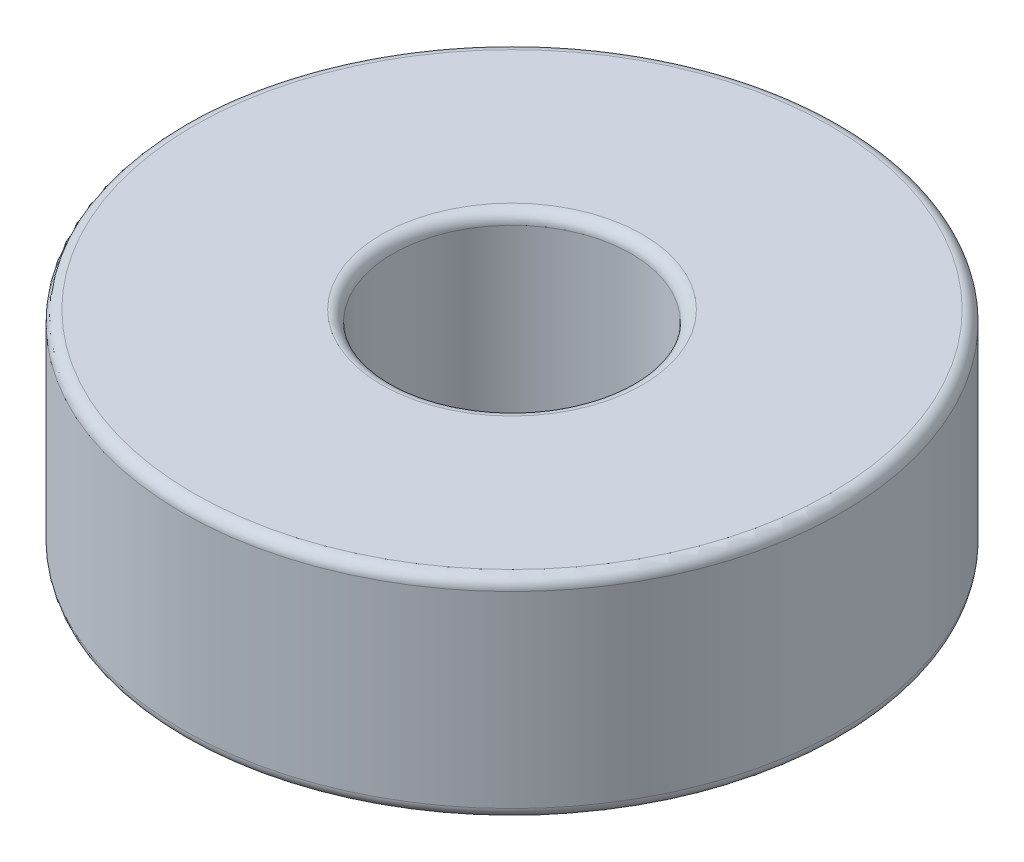
from build123d import *

# Parameters (mm, degrees)
SKETCH_1_R      = 23.5
SKETCH_1_R_2    = 8.5
EXTRUDE_1_DEPTH = 15
FILLET_1_R      = 0.8


with BuildPart() as part:
    # 草图1 → 拉伸1 (new body)
    with BuildSketch(Plane(origin=(0, 0, 0), x_dir=(1, 0, 0), z_dir=(0, 1, 0))):
        with Locations(Location((0, 0, 0), (0, 0, 270))):
            Circle(SKETCH_1_R)
        with Locations(Location((0, 0, 0), (0, 0, 270))):
            Circle(SKETCH_1_R_2, mode=Mode.SUBTRACT)
    extrude(amount=EXTRUDE_1_DEPTH)

    # 圆角1
    fillet_1_edges = [part.edges().sort_by_distance(p)[0] for p in [
        (0, 0, -23.5),
        (0, 15, -23.5),
        (0, 0, -8.5),
        (0, 15, -8.5),
    ]]
    fillet(fillet_1_edges, radius=FILLET_1_R)


solid = part.part
